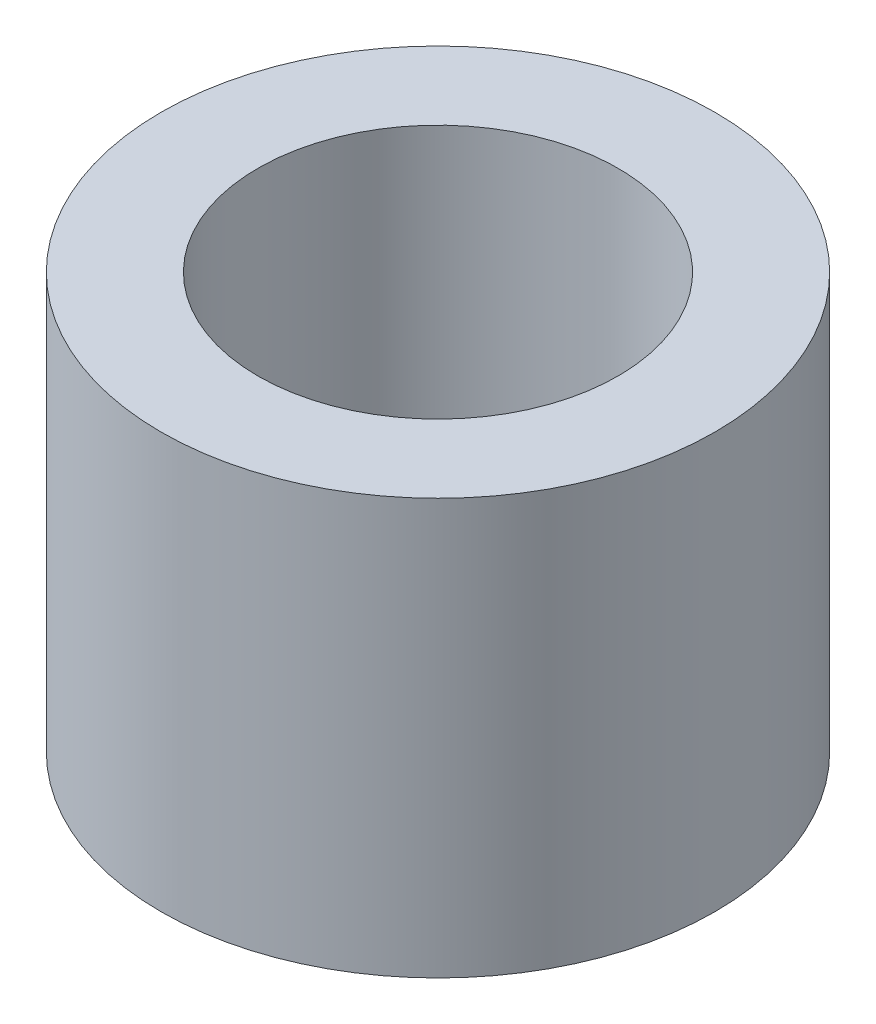
from build123d import *

# Parameters (mm, degrees)
SKETCH1_R           = 4
SKETCH1_R_2         = 2.6
BOSS_EXTRUDE1_DEPTH = 6


with BuildPart() as part:
    # Sketch1 → Boss-Extrude1 (new body)
    with BuildSketch(Plane(origin=(0, 0, 0), x_dir=(1, 0, 0), z_dir=(0, 1, 0))):
        with Locations(Location((0, 0, 0), (0, 0, 270))):
            Circle(SKETCH1_R)
        with Locations(Location((0, 0, 0), (0, 0, 270))):
            Circle(SKETCH1_R_2, mode=Mode.SUBTRACT)
    extrude(amount=BOSS_EXTRUDE1_DEPTH)


solid = part.part
